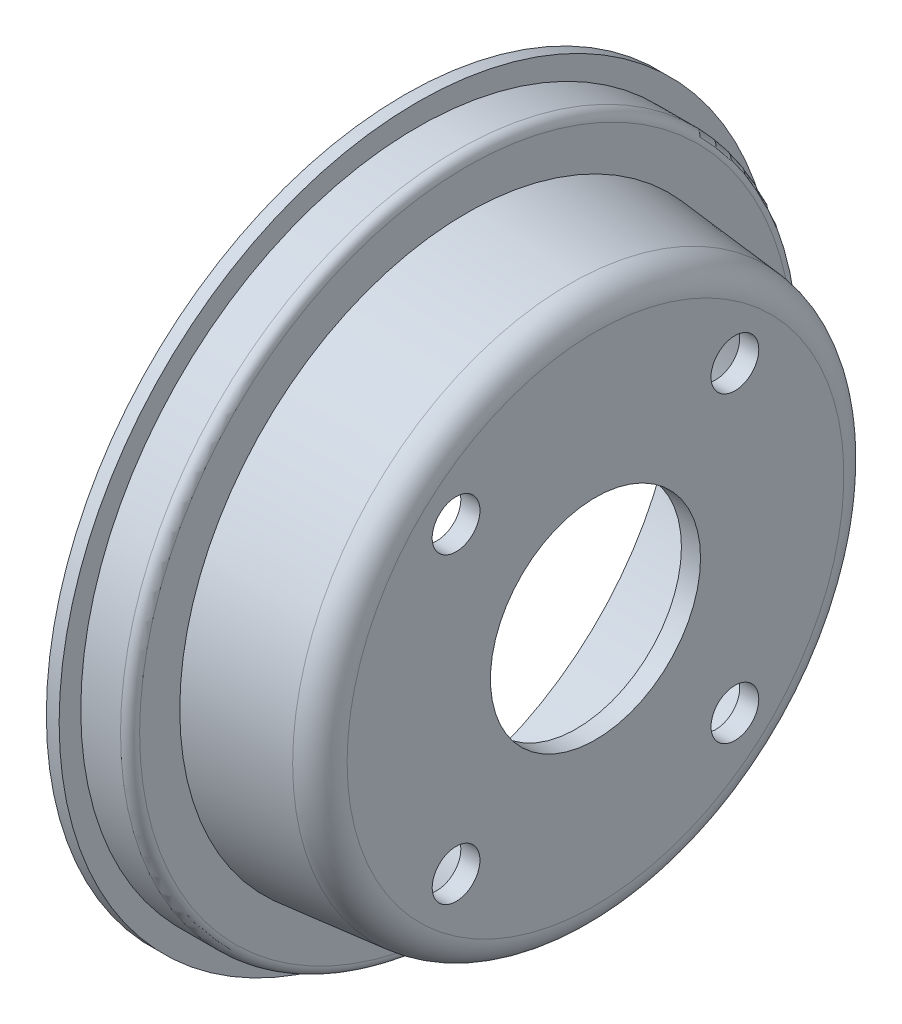
from build123d import *

# Parameters (mm, degrees)
SKETCH2_R          = 11
SKETCH2_R_2        = 2.5
CUT_EXTRUDE1_DEPTH = 10
FILLET1_R          = 3
FILLET2_R          = 1


with BuildPart() as part:
    # Sketch1 → Revolve1 (revolve)
    with BuildSketch(Plane.XY, mode=Mode.PRIVATE) as revolve1_sk:
        Polygon((-61.497364751, 54.207400123), (-61.497364751, 63.064837562), (-60.157873326, 63.064837562), (-60.157873326, 60.798367254), (-54.997364751, 60.798367254), (-54.997364751, 55.593672907), (-41.497364751, 54.299979424), (-41.497364751, 25.564837562), (-43.497364751, 25.564837562), (-43.497364751, 52.482475479), align=None)
    revolve(revolve1_sk.sketch.rotate(Axis((-61.497364751, 25.564837562, 0), (1, 0, 0)), 90), axis=Axis((-61.497364751, 25.564837562, 0), (1, 0, 0)))

    # Sketch2 → Cut-Extrude1 (cut)
    with BuildSketch(Plane(origin=(-41.497364751, 0, 0), x_dir=(0, 0, -1), z_dir=(1, 0, 0))):
        with Locations((0, 25.564837562)):
            Circle(SKETCH2_R)
        with Locations((-14.598664639, 41.420145509)):
            Circle(SKETCH2_R_2)
        with Locations((14.598664639, 41.420145509)):
            Circle(SKETCH2_R_2)
        with Locations((14.598664639, 9.709529615)):
            Circle(SKETCH2_R_2)
        with Locations((-14.598664639, 9.709529615)):
            Circle(SKETCH2_R_2)
    extrude(amount=-CUT_EXTRUDE1_DEPTH, mode=Mode.SUBTRACT)

    # Fillet1
    fillet1_edges = [part.edges().sort_by_distance(p)[0] for p in [
        (-41.497364751, 25.564837562, -28.735141862),
    ]]
    fillet(fillet1_edges, radius=FILLET1_R)

    # Fillet2
    fillet2_edges = [part.edges().sort_by_distance(p)[0] for p in [
        (-54.997364751, 25.564837562, -35.233529691),
    ]]
    fillet(fillet2_edges, radius=FILLET2_R)


solid = part.part
